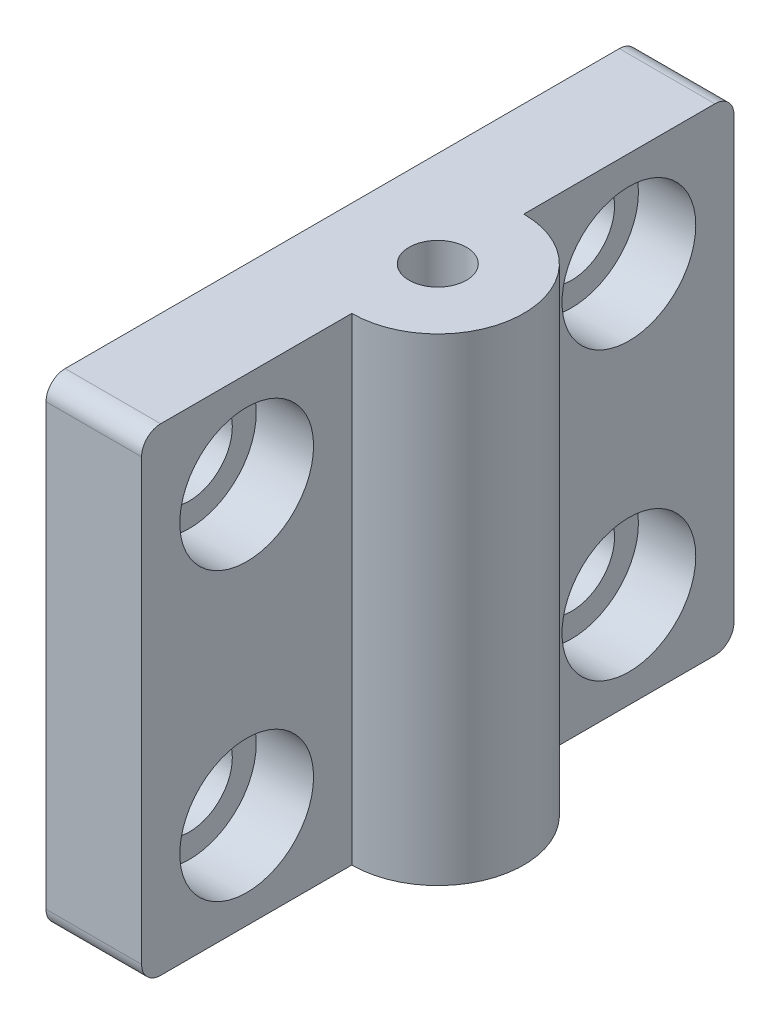
from build123d import *

# Parameters (mm, degrees)
SKETCH_1_R                   = 3
EXTRUDE_1_DEPTH              = 25
HOLE_WIZARD_M8_1_D           = 9
HOLE_WIZARD_M8_1_CBORE_D     = 14
HOLE_WIZARD_M8_1_CBORE_DEPTH = 6
FILLET_1_R                   = 2


with BuildPart() as part:
    # 草图1 → 凸台-拉伸1 (new, symmetric)
    with BuildSketch(Plane(origin=(0, 0, 0), x_dir=(1, 0, 0), z_dir=(0, 1, 0))):
        with BuildLine():
            Line((10, -9), (10, -31))
            Line((10, -31), (0, -31))
            Line((0, -31), (0, 31))
            Line((0, 31), (10, 31))
            Line((10, 31), (10, 9))
            ThreePointArc((10, 9), (19, 0), (10, -9))
        make_face()
        with Locations(Location((10, 0, 0), (0, 0, 270))):
            Circle(SKETCH_1_R, mode=Mode.SUBTRACT)
    extrude(amount=EXTRUDE_1_DEPTH, both=True)

    # M8 六角凹头螺钉的柱形沉头孔1 (through all)
    with Locations(Plane(origin=(10, 0, 0), x_dir=(0, 0, -1), z_dir=(1, 0, 0))):
        with Locations((-20, 15), (-20, -15), (20, -15), (20, 15)):
            CounterBoreHole(HOLE_WIZARD_M8_1_D / 2, HOLE_WIZARD_M8_1_CBORE_D / 2, HOLE_WIZARD_M8_1_CBORE_DEPTH)

    # 圆角1
    fillet_1_edges = [part.edges().sort_by_distance(p)[0] for p in [
        (5, 25, -31),
        (5, -25, -31),
        (5, 25, 31),
        (5, -25, 31),
    ]]
    fillet(fillet_1_edges, radius=FILLET_1_R)


solid = part.part
